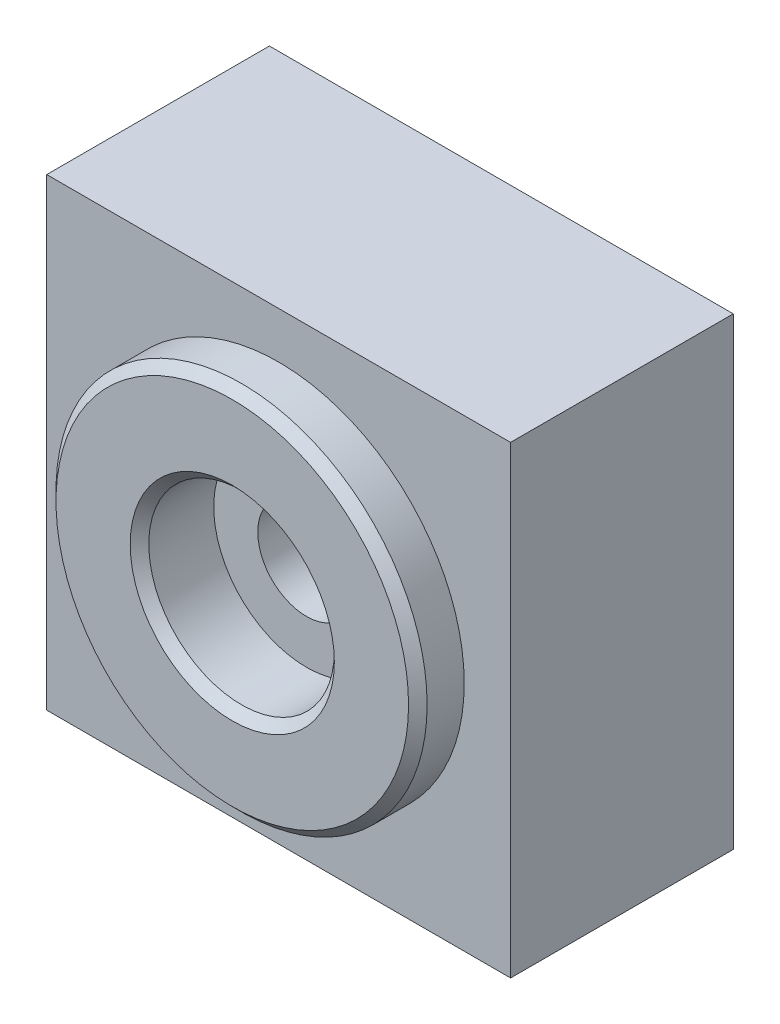
from build123d import *

# Parameters (mm, degrees)
SKETCH_1_W          = 50
SKETCH_1_H          = 50
EXTRUDE_1_DEPTH     = 29
SKETCH_3_R          = 10
CUT_EXTRUDE_1_DEPTH = 8
SKETCH_4_R          = 5.25
CUT_EXTRUDE_2_DEPTH = 21
CHAMFER_1_SIZE      = 1
SKETCH_5_OUTSIDE_W  = 67.286
SKETCH_5_OUTSIDE_H  = 67.286
SKETCH_5_OUTSIDE_R  = 20
CUT_EXTRUDE_3_DEPTH = 5
CHAMFER_2_SIZE      = 1


with BuildPart() as part:
    # 草图1 → 凸台-拉伸1 (new body)
    with BuildSketch(Plane.XY):
        Rectangle(SKETCH_1_W, SKETCH_1_H)
    extrude(amount=EXTRUDE_1_DEPTH)

    # 草图3 → 切除-拉伸1 (cut)
    with BuildSketch(Plane.XY.offset(29)):
        Circle(SKETCH_3_R)
    extrude(amount=-CUT_EXTRUDE_1_DEPTH, mode=Mode.SUBTRACT)

    # 草图4 → 切除-拉伸2 (cut)
    with BuildSketch(Plane(origin=(0, 0, 0), x_dir=(-1, 0, 0), z_dir=(0, 0, -1))):
        Circle(SKETCH_4_R)
    extrude(amount=-CUT_EXTRUDE_2_DEPTH, mode=Mode.SUBTRACT)

    # 倒角1
    chamfer_1_edges = [part.edges().sort_by_distance(p)[0] for p in [
        (-10, 0, 29),
    ]]
    chamfer(chamfer_1_edges, length=CHAMFER_1_SIZE)

    # 草图5 outside → 切除-拉伸3 (cut)
    with BuildSketch(Plane.XY.offset(29)):
        Rectangle(SKETCH_5_OUTSIDE_W, SKETCH_5_OUTSIDE_H)
        Circle(SKETCH_5_OUTSIDE_R, mode=Mode.SUBTRACT)
    extrude(amount=-CUT_EXTRUDE_3_DEPTH, mode=Mode.SUBTRACT)

    # 倒角2
    chamfer_2_edges = [part.edges().sort_by_distance(p)[0] for p in [
        (-20, 0, 29),
    ]]
    chamfer(chamfer_2_edges, length=CHAMFER_2_SIZE)


solid = part.part
